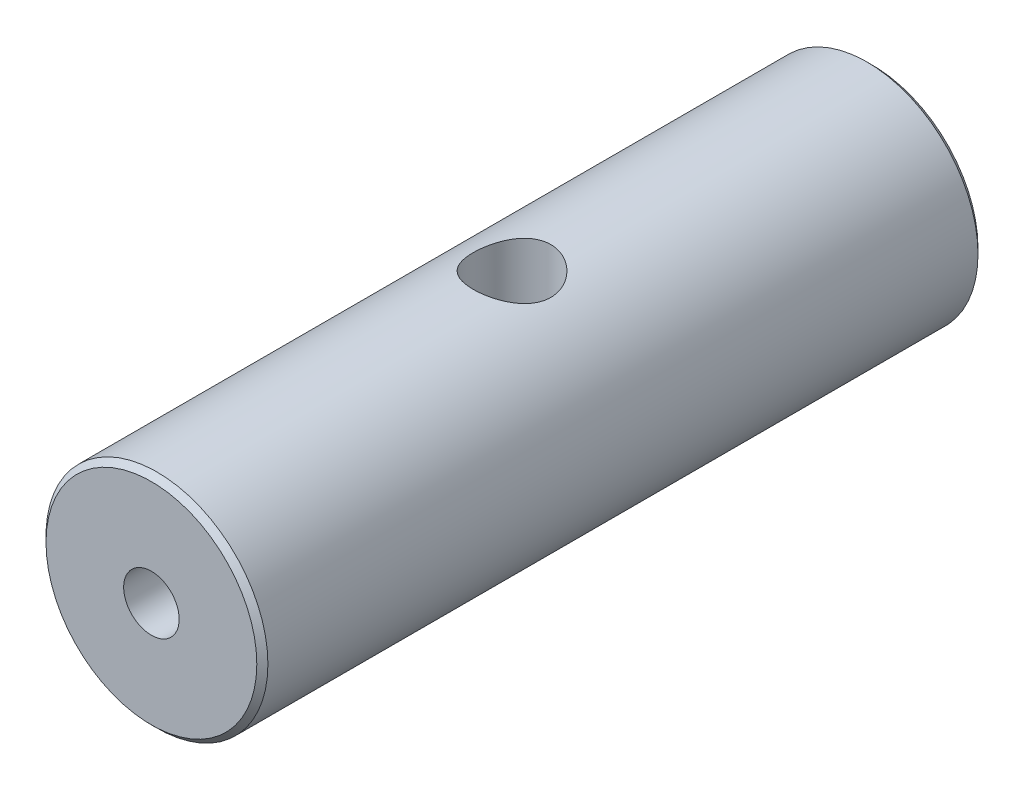
from build123d import *

# Parameters (mm, degrees)
SKETCH1_R               = 10
BOSS_EXTRUDE1_DEPTH     = 32.5
CHAMFER1_SIZE           = 0.5
M6_TAPPED_HOLE1_D       = 5
M6_TAPPED_HOLE1_DEPTH   = 15
M6_TAPPED_HOLE1_TIP     = 1.502151548
M6_TAPPED_HOLE2_D       = 5
M6_TAPPED_HOLE2_DEPTH   = 15
M6_TAPPED_HOLE2_TIP     = 1.502151548
CUT_EXTRUDE1_DEPTH      = 36.443617197
CUT_EXTRUDE1_DEPTH_BACK = 36.443617197
SKETCH8_R               = 3.5


with BuildPart() as part:
    # Sketch1 → Boss-Extrude1 (new, symmetric)
    with BuildSketch(Plane.XY):
        Circle(SKETCH1_R)
    extrude(amount=BOSS_EXTRUDE1_DEPTH, both=True)

    # Chamfer1
    chamfer1_edges = [part.edges().sort_by_distance(p)[0] for p in [
        (-10, 0, -32.5),
        (-10, 0, 32.5),
    ]]
    chamfer(chamfer1_edges, length=CHAMFER1_SIZE)

    # M6 Tapped Hole1
    with Locations(Plane.XY.offset(32.5)):
        with Locations((0, 0)):
            Hole(M6_TAPPED_HOLE1_D / 2, depth=M6_TAPPED_HOLE1_DEPTH)
            with Locations((0, 0, -(M6_TAPPED_HOLE1_DEPTH + M6_TAPPED_HOLE1_TIP / 2))):  # 118° drill point
                Cone(0, M6_TAPPED_HOLE1_D / 2, M6_TAPPED_HOLE1_TIP, mode=Mode.SUBTRACT)

    # M6 Tapped Hole2
    with Locations(Plane(origin=(0, 0, -32.5), x_dir=(-1, 0, 0), z_dir=(0, 0, -1))):
        with Locations((0, 0)):
            Hole(M6_TAPPED_HOLE2_D / 2, depth=M6_TAPPED_HOLE2_DEPTH)
            with Locations((0, 0, -(M6_TAPPED_HOLE2_DEPTH + M6_TAPPED_HOLE2_TIP / 2))):  # 118° drill point
                Cone(0, M6_TAPPED_HOLE2_D / 2, M6_TAPPED_HOLE2_TIP, mode=Mode.SUBTRACT)

    # Sketch8 → Cut-Extrude1 (cut, two sides: drawn at the far end of the back side and taken through both)
    with BuildSketch(Plane(origin=(0, 0, 0), x_dir=(1, 0, 0), z_dir=(0, 1, 0)).offset(-CUT_EXTRUDE1_DEPTH_BACK)):
        with Locations(Location((0, 0, 0), (0, 0, 270))):
            Circle(SKETCH8_R)
    extrude(amount=CUT_EXTRUDE1_DEPTH + CUT_EXTRUDE1_DEPTH_BACK, mode=Mode.SUBTRACT)


solid = part.part
